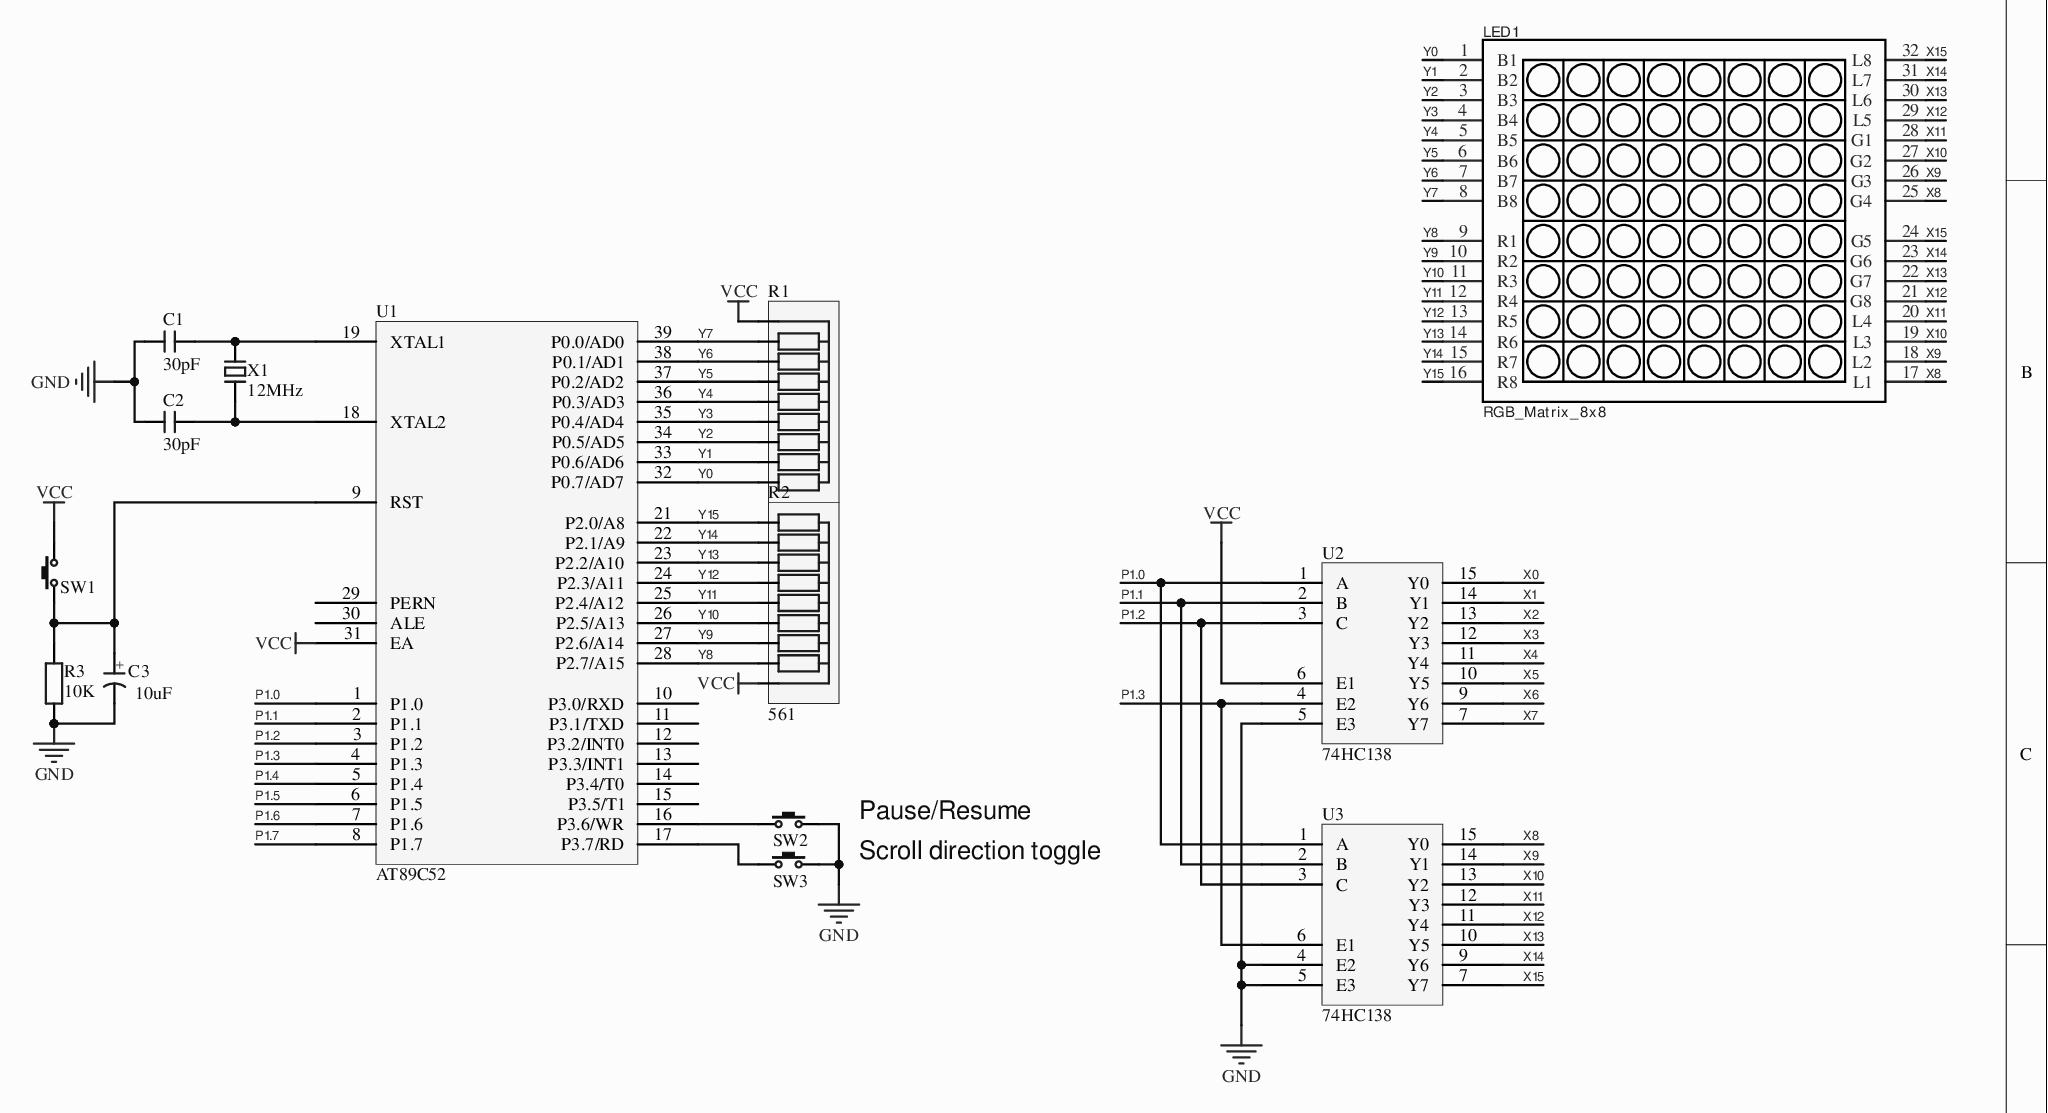
[diagram p0: MISC80553-4.SchDoc]
# Altium project MISC80553-7.PrjPcb
1 sheet, 14 parts. Net scope: global (net labels, ports and power ports of the same name join across sheets).
Board file: MISC80553.PcbDoc

## Sheet MISC80553-4.SchDoc
size A4; SheetNumber: 1; SheetTotal: 1

### Parts
C1  30pF  [CC 1.8*3.6]
C2  30pF  [CC 1.8*3.6]
C3  10uF  [CAP 1.5*4*8]
LED1  RGB_Matrix_8x8  [RGB_MATRIX_8X8]
R1  561  [R SIP9-2.54]
R2  561  [R SIP9-2.54]
R3  10K  [RS 1/8W]
SW1  3x6x5  [TSW DIP-3*6*5]  (value not drawn)
SW2  3x6x5  [TSW DIP-3*6*5]  (value not drawn)
SW3  3x6x5  [TSW DIP-3*6*5]  (value not drawn)
U1  AT89C52  [DIP40]
U2  74HC138  [648-08]
U3  74HC138  [648-08]
X1  12MHz  [OSC HC-49S]

### Nets
GND: C1.1 C2.1 C3.2(K) R3.1 SW2.2 SW3.2 U2.5(E3) U3.4(E2) U3.5(E3)
VCC: R1.1 R2.1 SW1.2 U1.31(EA) U2.6(E1)
P1.0: U1.1(P1.0) U2.1(A) U3.1(A)
P1.1: U1.2(P1.1) U2.2(B) U3.2(B)
P1.2: U1.3(P1.2) U2.3(C) U3.3(C)
P1.3: U1.4(P1.3) U2.4(E2) U3.6(E1)
P1.4: U1.5(P1.4)
P1.5: U1.6(P1.5)
P1.6: U1.7(P1.6)
P1.7: U1.8(P1.7)
X0: U2.15(Y0)
X1: U2.14(Y1)
X2: U2.13(Y2)
X3: U2.12(Y3)
X4: U2.11(Y4)
X5: U2.10(Y5)
X6: U2.9(Y6)
X7: U2.7(Y7)
X8: LED1.17(L1) LED1.25(G4) U3.15(Y0)
X9: LED1.18(L2) LED1.26(G3) U3.14(Y1)
X10: LED1.19(L3) LED1.27(G2) U3.13(Y2)
X11: LED1.20(L4) LED1.28(G1) U3.12(Y3)
X12: LED1.21(G8) LED1.29(L5) U3.11(Y4)
X13: LED1.22(G7) LED1.30(L6) U3.10(Y5)
X14: LED1.23(G6) LED1.31(L7) U3.9(Y6)
X15: LED1.24(G5) LED1.32(L8) U3.7(Y7)
Y0: LED1.1(B1) R1.9 U1.32(P0.7/AD7)
Y1: LED1.2(B2) R1.8 U1.33(P0.6/AD6)
Y2: LED1.3(B3) R1.7 U1.34(P0.5/AD5)
Y3: LED1.4(B4) R1.6 U1.35(P0.4/AD4)
Y4: LED1.5(B5) R1.5 U1.36(P0.3/AD3)
Y5: LED1.6(B6) R1.4 U1.37(P0.2/AD2)
Y6: LED1.7(B7) R1.3 U1.38(P0.1/AD1)
Y7: LED1.8(B8) R1.2 U1.39(P0.0/AD0)
Y8: LED1.9(R1) R2.2 U1.28(P2.7/A15)
Y9: LED1.10(R2) R2.3 U1.27(P2.6/A14)
Y10: LED1.11(R3) R2.4 U1.26(P2.5/A13)
Y11: LED1.12(R4) R2.5 U1.25(P2.4/A12)
Y12: LED1.13(R5) R2.6 U1.24(P2.3/A11)
Y13: LED1.14(R6) R2.7 U1.23(P2.2/A10)
Y14: LED1.15(R7) R2.8 U1.22(P2.1/A9)
Y15: LED1.16(R8) R2.9 U1.21(P2.0/A8)
NetC1_2: C1.2 U1.19(XTAL1) X1.2
NetC2_2: C2.2 U1.18(XTAL2) X1.1
NetC3_1: C3.1(A) R3.2 SW1.1 U1.9(RST)
NetSW2_1: SW2.1 U1.16(P3.6/WR)
NetSW3_1: SW3.1 U1.17(P3.7/RD)

Not connected (* = marked no-connect by the designer): U1 10(P3.0/RXD) 11(P3.1/TXD) 12(P3.2/INT0) 13(P3.3/INT1) 14(P3.4/T0) 15(P3.5/T1) 29(PERN) 30(ALE)

### Notes on the sheet
- Pause/Resume
- Scroll direction toggle

### Library data of the parts
C1 C2 = C: Non-polar SMD capacitor; 版权归属: COMPANY_A; BOM名称: Non-polar SMD capacitor
C3 = C-CAP: THT electrolytic capacitor; 版权归属: COMPANY_A; BOM名称: THT electrolytic capacitor
R1 R2 = R SIP9: Single in-line resistor array; 版权归属: COMPANY_A; BOM名称: Single in-line resistor array
R3 = R: SMD resistor; 版权归属: COMPANY_A; BOM名称: SMD resistor
SW1-SW3 = TSW 3x6: 3x6 tact switch; 版权归属: COMPANY_A; BOM名称: 3x6 tact switch
U2 U3 = Component_1
X1 = XTAL-2P: 2-pin passive crystal; BOM名称: 2-pin passive crystal